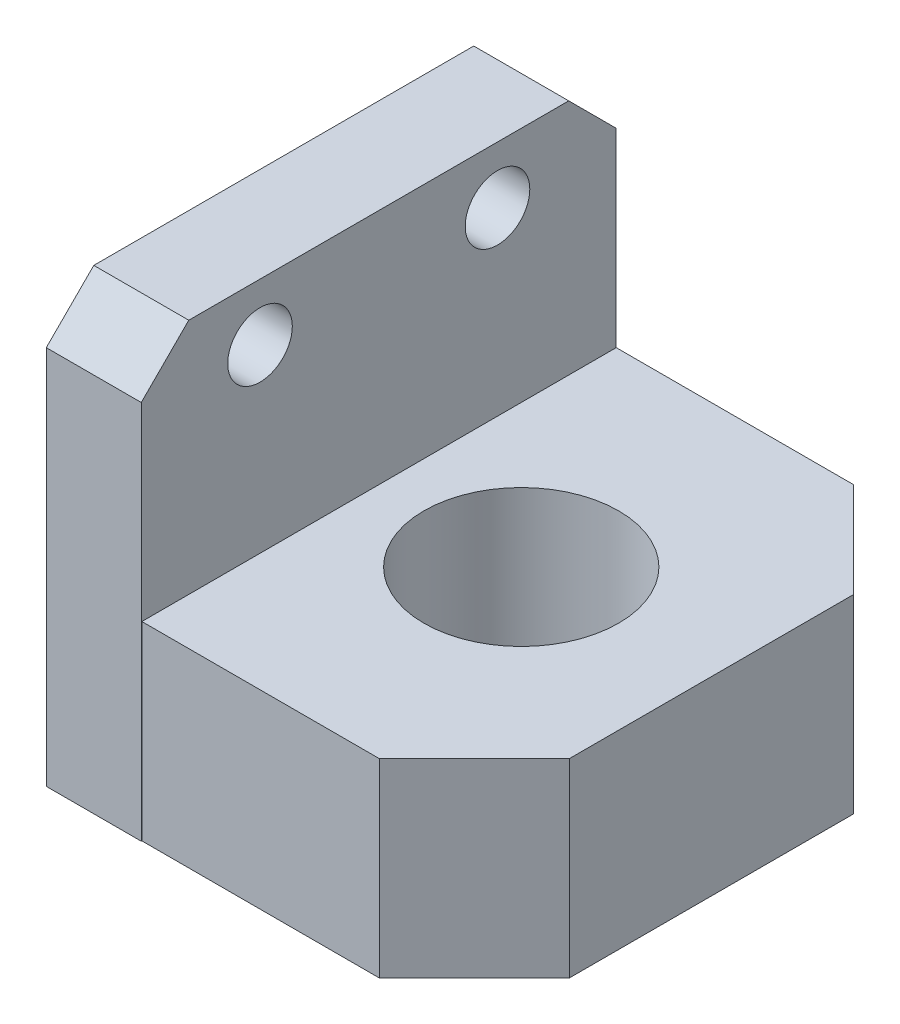
from build123d import *

# Parameters (mm, degrees)
SKETCH_1_W                  = 50
SKETCH_1_H                  = 45
EXTRUDE_1_DEPTH             = 10
SKETCH_2_W                  = 49.938204031
SKETCH_2_H                  = 20
EXTRUDE_2_DEPTH             = 35
HOLE_WIZARD_20_5_20_5_1_D   = 20.5
SKETCH_6_W                  = 3.4
SKETCH_6_H                  = 10
HOLE_WIZARD_M8_1_AT_2_COUNT = 2
HOLE_WIZARD_M8_1_AT_2_PITCH = 25
HOLE_WIZARD_M8_1_AT_3_COUNT = 2
HOLE_WIZARD_M8_1_AT_3_PITCH = 30
HOLE_WIZARD_M8_1_AT_4_COUNT = 2
HOLE_WIZARD_M8_1_AT_4_PITCH = 39.05124838
CHAMFER_1_SIZE              = 10
CHAMFER_2_SIZE              = 5


with BuildPart() as part:
    # 草图1 → 凸台-拉伸1 (new body)
    with BuildSketch(Plane(origin=(0, 0, 0), x_dir=(0, 0, -1), z_dir=(1, 0, 0))):
        Rectangle(SKETCH_1_W, SKETCH_1_H)
    extrude(amount=EXTRUDE_1_DEPTH)

    # 草图2 → 凸台-拉伸2 (add)
    with BuildSketch(Plane(origin=(10, 0, 0), x_dir=(0, 0, -1), z_dir=(1, 0, 0))):
        with Locations((0.030897984, -12.5)):
            Rectangle(SKETCH_2_W, SKETCH_2_H)
    extrude(amount=EXTRUDE_2_DEPTH)

    # Ø20.5 (20.5) 直径孔1 (through all)
    with Locations(Plane(origin=(0, -22.5, 0), x_dir=(-1, 0, 0), z_dir=(0, -1, 0))):
        with Locations((-25, 0)):
            Hole(HOLE_WIZARD_20_5_20_5_1_D / 2)

    # 草图6 → M8 螺纹孔1 (revolve, cut)
    with BuildSketch(Plane(origin=(10, 16.5, 12.5), x_dir=(0, 0, -1), z_dir=(0, 1, 0))):
        with Locations((1.7, 5)):
            Rectangle(SKETCH_6_W, SKETCH_6_H)
    hole_wizard_m8_1 = revolve(axis=Axis((16.35, 16.5, 12.5), (-1, 0, 0)), mode=Mode.SUBTRACT)

    # M8 螺纹孔1 at 2: M8 螺纹孔1 ×2
    with Locations(*[(0, 0, -i * HOLE_WIZARD_M8_1_AT_2_PITCH) for i in range(1, HOLE_WIZARD_M8_1_AT_2_COUNT)]):
        add(hole_wizard_m8_1, mode=Mode.SUBTRACT)

    # M8 螺纹孔1 at 3: M8 螺纹孔1 ×2
    with Locations(*[(0, -i * HOLE_WIZARD_M8_1_AT_3_PITCH, 0) for i in range(1, HOLE_WIZARD_M8_1_AT_3_COUNT)]):
        add(hole_wizard_m8_1, mode=Mode.SUBTRACT)

    # M8 螺纹孔1 at 4: M8 螺纹孔1 ×2
    with Locations(*[Vector(0, -0.7682212795973759, -0.64018439966448) * (i * HOLE_WIZARD_M8_1_AT_4_PITCH) for i in range(1, HOLE_WIZARD_M8_1_AT_4_COUNT)]):
        add(hole_wizard_m8_1, mode=Mode.SUBTRACT)

    # 倒角1
    chamfer_1_edges = [part.edges().sort_by_distance(p)[0] for p in [
        (45, -12.5, -25),
        (45, -12.5, 24.938204031),
    ]]
    chamfer(chamfer_1_edges, length=CHAMFER_1_SIZE)

    # 倒角2
    chamfer_2_edges = [part.edges().sort_by_distance(p)[0] for p in [
        (5, 22.5, 25),
        (5, 22.5, -25),
    ]]
    chamfer(chamfer_2_edges, length=CHAMFER_2_SIZE)


solid = part.part
